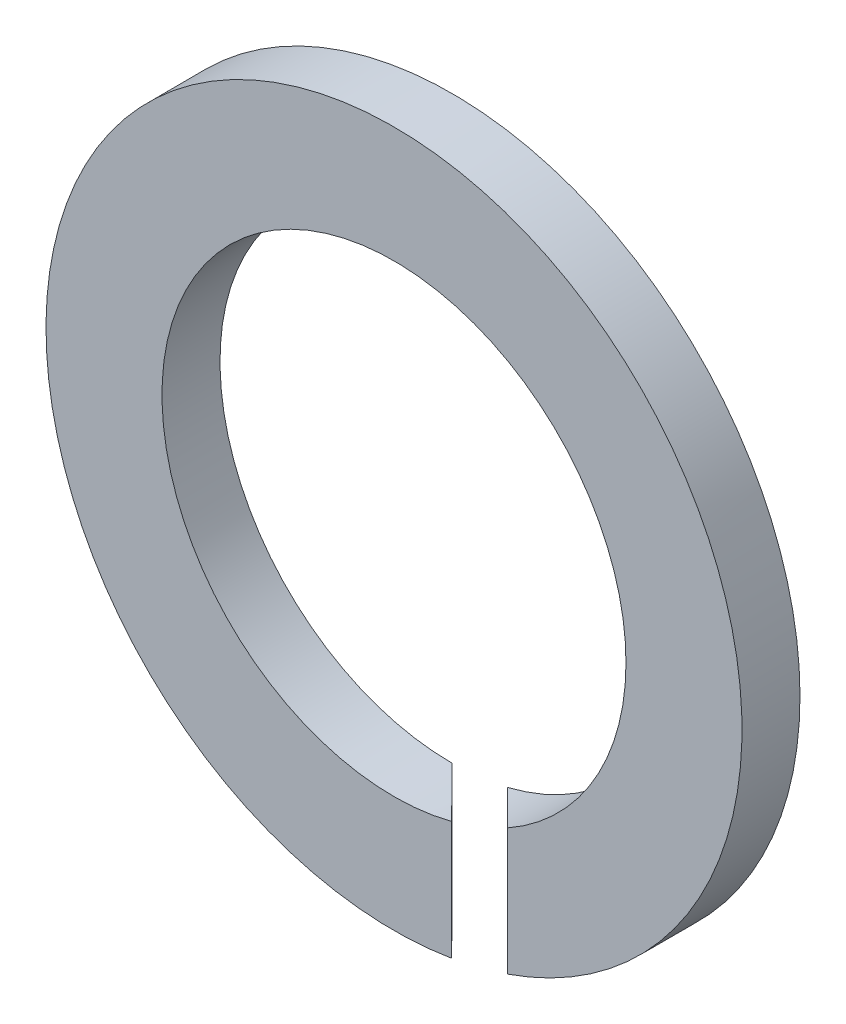
from build123d import *

# Parameters (mm, degrees)
SKETCH1_R           = 6
SKETCH1_R_2         = 4
BOSS_EXTRUDE1_DEPTH = 1
CUT_EXTRUDE1_DEPTH  = 9.544003745


with BuildPart() as part:
    # Sketch1 → Boss-Extrude1 (new body)
    with BuildSketch(Plane.XY):
        Circle(SKETCH1_R)
        Circle(SKETCH1_R_2, mode=Mode.SUBTRACT)
    extrude(amount=BOSS_EXTRUDE1_DEPTH)

    # Sketch2 → Cut-Extrude1 (cut, through all)
    with BuildSketch(Plane(origin=(0, 0, 0), x_dir=(1, 0, 0), z_dir=(0, 1, 0))):
        Polygon((0, 0), (0.95899064, 0), (1.953022833, -1), (0.994032193, -1), align=None)
    extrude(amount=-CUT_EXTRUDE1_DEPTH, mode=Mode.SUBTRACT)


solid = part.part
